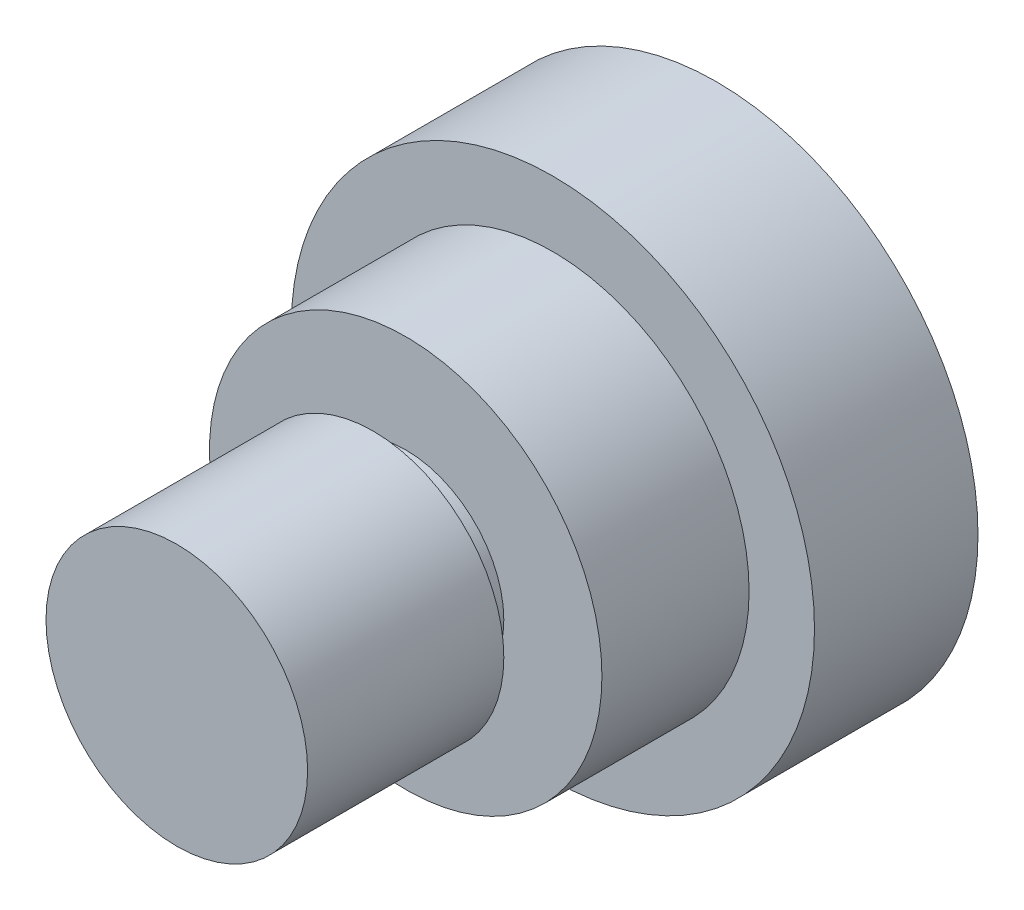
SolidWorks part; units mm, degrees
material "20#"
ref_plane "Front Plane" through (0, 0, 0) normal (0, 0, 1) x (1, 0, 0)
ref_plane "Top Plane" through (0, 0, 0) normal (0, 1, 0) x (1, 0, 0)
ref_plane "Right Plane" through (0, 0, 0) normal (1, 0, 0) x (0, 0, -1)
sketch "Sketch1" plane through (0, 0, 0) normal (1, 0, 0) x (0, 0, -1)
  line L0 (0, 0) -> (16.5, 0) construction
  line L1 (16.5, 0) -> (16.5, 8)
  line L2 (16.5, 8) -> (11.5, 8)
  line L3 (11.5, 8) -> (11.5, 6)
  line L4 (11.5, 6) -> (7, 6)
  line L5 (7, 6) -> (7, 3)
  line L6 (6, 4) -> (0, 4)
  line L7 (0, 4) -> (0, 0)
  line L8 (0, 0) -> (16.5, 0)
  line L9 (7, 3) -> (6, 3)
  line L10 (6, 3) -> (6, 4)
  dimension "D1" = 16.5
  dimension "D2" = 5
  dimension "D3" = 4.5
  dimension "D4" = 7
  dimension "D5" = 8
  dimension "D6" = 12
  dimension "D7" = 16
  dimension "D8" = 1
  dimension "D9" = 1
revolve "Revolve1" add sketch "Sketch1" angle 360 about L0
cosmetic thread "Cosmetic Thread1" parameters "D2"=6.647
